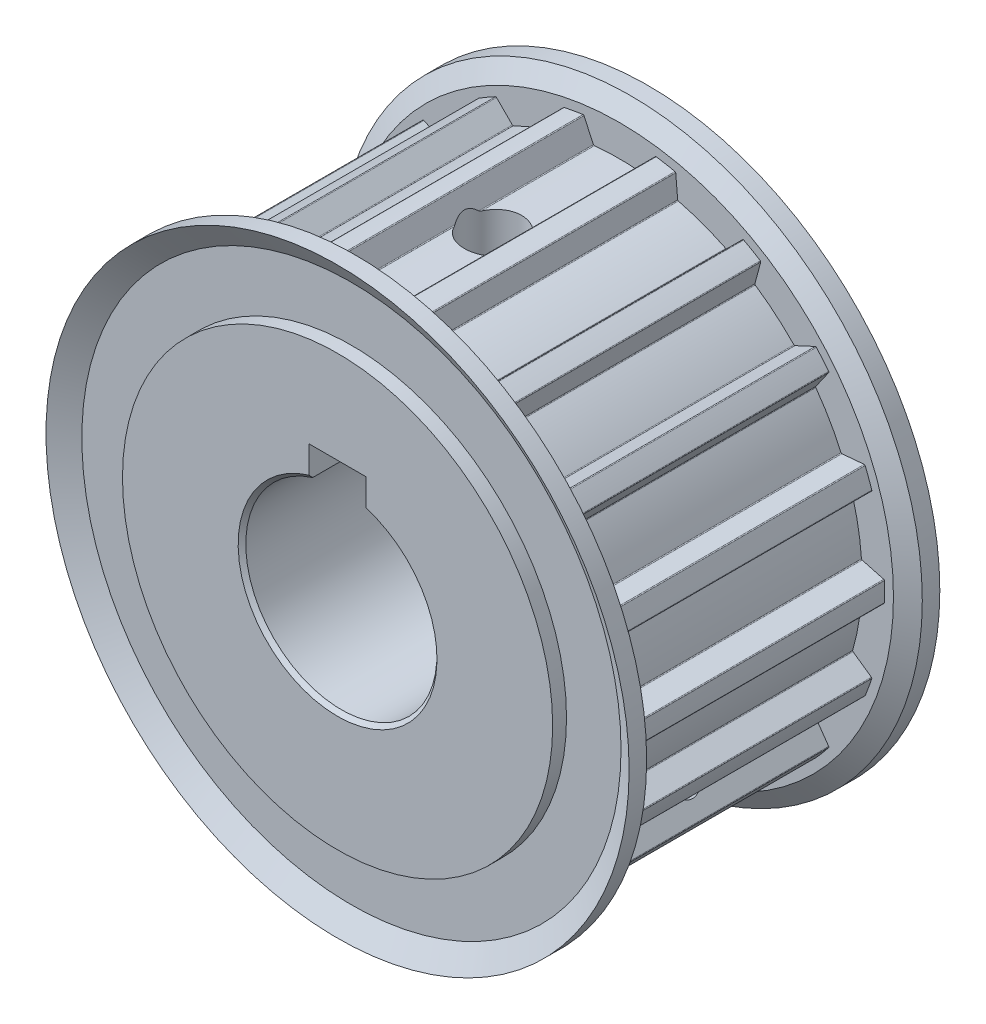
from build123d import *

# Parameters (mm, degrees)
BOSS_EXTRUDE1_DEPTH     = 13.25
CIRPATTERN1_COUNT       = 18
CUT_EXTRUDE2_DEPTH      = 47.092976688
CUT_EXTRUDE2_DEPTH_BACK = 47.092976688
CHAMFER2_SIZE           = 0.4
CUT_EXTRUDE3_START      = 12.8
SKETCH15_R              = 3
CUT_EXTRUDE3_DEPTH      = 34.292976688
SKETCH16_R              = 3
CUT_EXTRUDE4_DEPTH      = 47.092976688


with BuildPart() as part:
    # Sketch3 → Revolve1 (revolve)
    with BuildSketch(Plane(origin=(0, 0, 0), x_dir=(0, 0, -1), z_dir=(1, 0, 0)), mode=Mode.PRIVATE) as revolve1_sk:
        Polygon((16.25, 0), (16.25, 22.5), (14.8, 22.5), (14.8, 28.201883636), (16.25, 30.5), (14.417260302, 30.5), (13.25, 28.65), (13.25, 25.365), (-13.25, 25.365), (-13.25, 28.65), (-14.417260302, 30.5), (-16.25, 30.5), (-14.8, 28.201883636), (-14.8, 22.5), (-16.25, 22.5), (-16.25, 0), align=None)
    revolve(revolve1_sk.sketch.rotate(Axis((0, 0, 16.25), (0, 0, -1)), 90), axis=Axis((0, 0, 16.25), (0, 0, -1)))

    # Sketch4 → Boss-Extrude1 (add, symmetric)
    with BuildSketch(Plane.XY):
        with BuildLine():
            Line((2.735168051, 25.285048485), (3.722692974, 27.402802518))
            ThreePointArc((3.722692974, 27.402802518), (3.76555756, 27.448395065), (3.82712764, 27.459583373))
            ThreePointArc((3.82712764, 27.459583373), (4.814395726, 27.303794952), (5.795407039, 27.11252261))
            ThreePointArc((5.795407039, 27.11252261), (5.849437362, 27.080950831), (5.874123327, 27.0234473))
            Line((5.874123327, 27.0234473), (6.077778673, 24.695656047))
            ThreePointArc((6.077778673, 24.695656047), (6.101335395, 24.639452761), (6.153139756, 24.607358577))
            ThreePointArc((6.153139756, 24.607358577), (4.404586027, 24.979648655), (2.634152284, 25.227851013))
            ThreePointArc((2.634152284, 25.227851013), (2.693809317, 25.240291546), (2.735168051, 25.285048485))
        make_face()
    boss_extrude1 = extrude(amount=BOSS_EXTRUDE1_DEPTH, both=True)

    # CirPattern1: Boss-Extrude1 ×18 about axis
    cirpattern1_axis = Axis((0, 0, 0), (0, 0, 1))
    for i in range(1, CIRPATTERN1_COUNT):
        add(boss_extrude1.rotate(cirpattern1_axis, i * 360 / CIRPATTERN1_COUNT))

    # Sketch9 → Cut-Extrude2 (cut, two sides: drawn at the far end of the back side and taken through both)
    with BuildSketch(Plane.XY.offset(-CUT_EXTRUDE2_DEPTH_BACK)):
        with BuildLine():
            Line((-3, 9.539392014), (-3, 12.8))
            Line((-3, 12.8), (3, 12.8))
            Line((3, 12.8), (3, 9.539392014))
            ThreePointArc((3, 9.539392014), (0, -10), (-3, 9.539392014))
        make_face()
    extrude(amount=CUT_EXTRUDE2_DEPTH + CUT_EXTRUDE2_DEPTH_BACK, mode=Mode.SUBTRACT)

    # Chamfer2
    chamfer2_edges = [part.edges().sort_by_distance(p)[0] for p in [
        (0, -10, -16.25),
        (0, -10, 16.25),
    ]]
    chamfer(chamfer2_edges, length=CHAMFER2_SIZE)

    # Sketch15 → Cut-Extrude3 (cut, through all)
    with BuildSketch(Plane(origin=(0, 0, 0), x_dir=(1, 0, 0), z_dir=(0, 1, 0)).offset(CUT_EXTRUDE3_START)):
        with Locations(Location((0, 0, 0), (0, 0, 28.591885504))):
            Circle(SKETCH15_R)
    extrude(amount=CUT_EXTRUDE3_DEPTH, mode=Mode.SUBTRACT)

    # Sketch16 → Cut-Extrude4 (cut, through all)
    with BuildSketch(Plane(origin=(0, 0, 0), x_dir=(-0.499999999999998, -0.8660254037844398, 0), z_dir=(-0.8660254037844398, 0.499999999999998, 0))):
        Circle(SKETCH16_R)
    extrude(amount=-CUT_EXTRUDE4_DEPTH, mode=Mode.SUBTRACT)


solid = part.part
